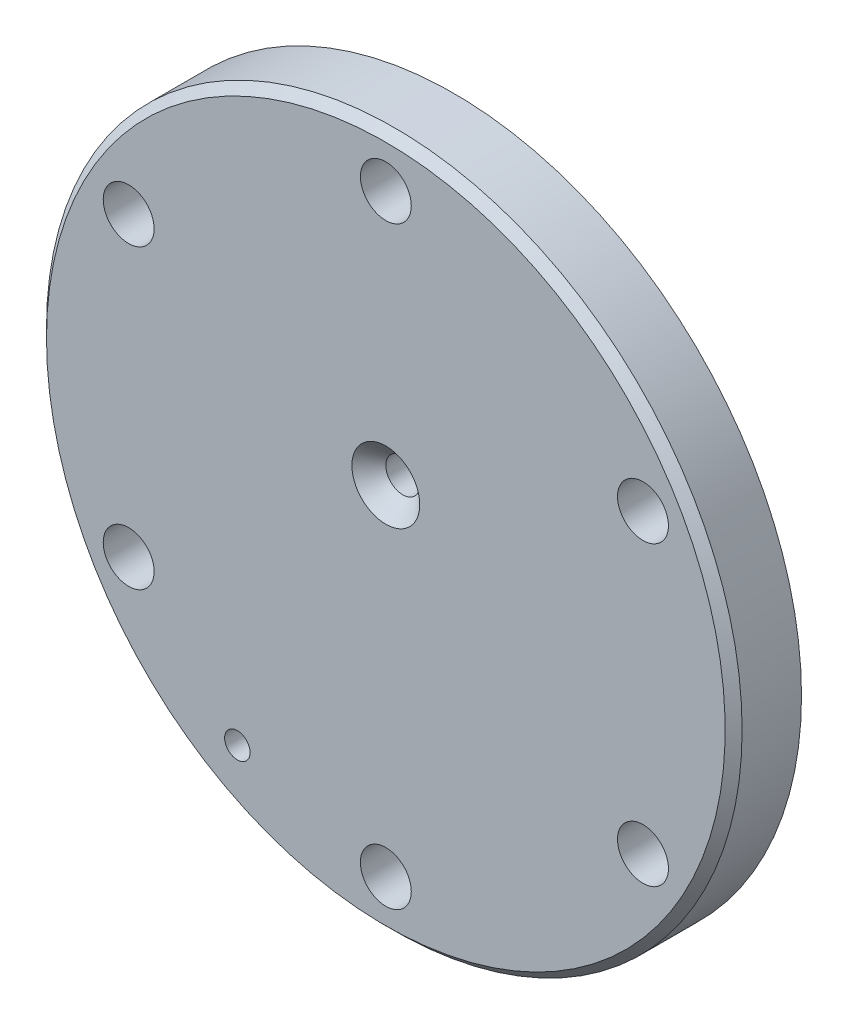
SolidWorks part; units mm, degrees
ref_plane "Front Plane" through (0, 0, 0) normal (0, 0, 1) x (1, 0, 0)
ref_plane "Top Plane" through (0, 0, 0) normal (0, 1, 0) x (1, 0, 0)
ref_plane "Right Plane" through (0, 0, 0) normal (1, 0, 0) x (0, 0, -1)
other "Configuration Table"
sketch "Sketch1" plane through (0, 0, 0) normal (1, 0, 0) x (0, 0, -1)
  line L0 (0, 0) -> (0, 24)
  line L1 (0, 24) -> (-2, 24)
  line L2 (-2, 24) -> (-2, 41)
  line L3 (-2, 41) -> (-10, 41)
  line L4 (-10, 41) -> (-10, 0)
  line L5 (-10, 0) -> (0, 0)
  line L6 (-25.9375, 0) -> (22.6042, 0) construction
  dimension "D1" = 10
  dimension "D2" = 24
  dimension "D3" = 41
  dimension "D4" = 2
revolve "Revolve1" add sketch "Sketch1" angle 360 about L6
sketch "Sketch2" plane through (0, 0, 2) normal (0, 0, -1) x (-1, 0, 0)
  line L0 (-45.8475, 0) -> (59.8236, 0) construction
  line L1 (0, 43.5921) -> (0, -44.4055) construction
  line L2 (0, 0) -> (23.7197, -41.0838) construction
  circle A0 centre (0, 0) radius 35 construction
  circle A1 centre (0, 35) radius 3
  circle A2 centre (30.3109, 17.5) radius 3
  circle A3 centre (30.3109, -17.5) radius 3
  circle A4 centre (0, -35) radius 3
  circle A5 centre (-30.3109, -17.5) radius 3
  circle A6 centre (-30.3109, 17.5) radius 3
  circle A7 centre (17.5, -30.3109) radius 1.5
  circle A8 centre (0, 5) radius 2
  point P21 (0, 0)
  dimension "D1" = 70
  dimension "D2" = 6
  dimension "D4" = 3
  dimension "D6" = 4
  dimension "D3" = 30
  dimension "D5" = 5
extrude "Cut-Extrude1" cut sketch "Sketch2" against normal through all and the other way blind 10
chamfer "Chamfer1" distance 1 angle 45 1 edges at (41, 0, 10)
chamfer "Chamfer2" distance 2 angle 45 1 edges at (-2, 5, 10)
